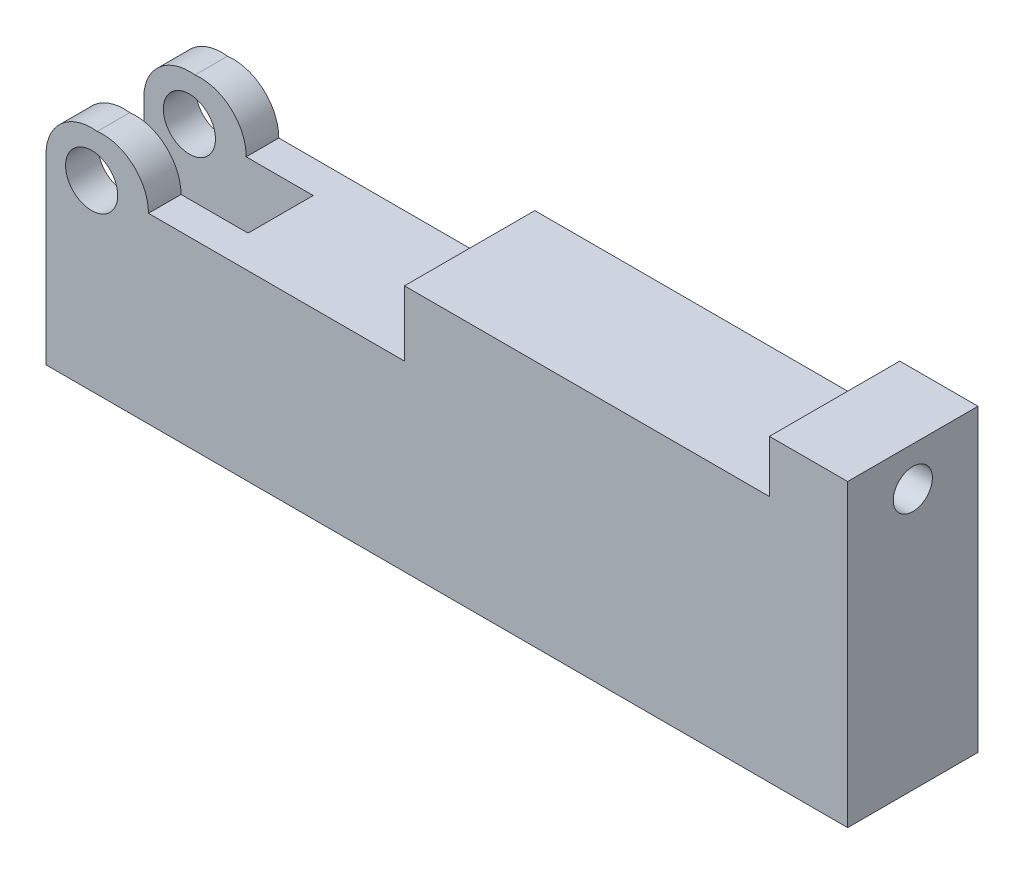
SolidWorks part; units mm, degrees
ref_plane "前视基准面" through (0, 0, 0) normal (0, 0, 1) x (1, 0, 0)
ref_plane "上视基准面" through (0, 0, 0) normal (0, 1, 0) x (1, 0, 0)
ref_plane "右视基准面" through (0, 0, 0) normal (1, 0, 0) x (0, 0, -1)
sketch "草图1" plane through (0, 0, 0) normal (0, 0, 1) x (1, 0, 0)
  line L0 (0.9754, 10.251) -> (6.9754, 10.251)
  line L1 (6.9754, 10.251) -> (6.9754, -12.749)
  line L2 (6.9754, -12.749) -> (-54.5246, -12.749)
  line L4 (-27.0246, 6.251) -> (0.9754, 6.251)
  line L5 (0.9754, 6.251) -> (0.9754, 10.251)
  line L6 (-51.0246, 4.751) -> (-50.1646, 4.751)
  line L7 (-54.5246, 1.251) -> (-54.5246, -12.749)
  line L8 (-46.6646, 1.251) -> (-27.0246, 1.251)
  line L9 (-27.0246, 1.251) -> (-27.0246, 6.251)
  circle A0 centre (-51.0246, 1.251) radius 2
  arc A2 (-50.5946, 4.7245) -> (-54.5246, 1.251) centre (-51.0246, 1.251) ccw
  arc A3 (-46.6646, 1.251) -> (-50.5946, 4.7245) centre (-50.1646, 1.251) ccw
  dimension "D5" = 4
  dimension "D8" = 7
  dimension "D1" = 23
  dimension "D2" = 4
  dimension "D4" = 6
  dimension "D6" = 5
  dimension "D9" = 0.86
extrude "凸台-拉伸1" add sketch "草图1" along normal blind 10 contours L8 A3 A2 L7 L2 L1 L0 L5 L4 L9 A0
sketch "草图2" plane through (6.9754, 0, 0) normal (1, 0, 0) x (0, 0, -1)
  line L0 (0, 10.251) -> (0, -12.749) construction
  line L1 (-10, 10.251) -> (0, 10.251) construction
  circle A0 centre (-5, 7.251) radius 1.5
  dimension "D3" = 3
  dimension "D1" = 5
  dimension "D2" = 3
extrude "切除-拉伸1" cut sketch "草图2" against normal blind 6
sketch "草图3" plane through (-54.5246, 0, 0) normal (-1, 0, 0) x (0, 0, 1)
  line L3 (2.5, 4.751) -> (7.5, 4.751)
  line L5 (10, 4.751) -> (0, 4.751) construction
  line L7 (2.5, 4.751) -> (2.5, -4.249)
  line L8 (2.5, -4.249) -> (7.5, -4.249)
  line L9 (7.5, -4.249) -> (7.5, 4.751)
  line L10 (0, 1.251) -> (0, -12.749) construction
  dimension "D1" = 2.5
  dimension "D2" = 5
  dimension "D3" = 9
extrude "切除-拉伸2" cut sketch "草图3" against normal blind 13
